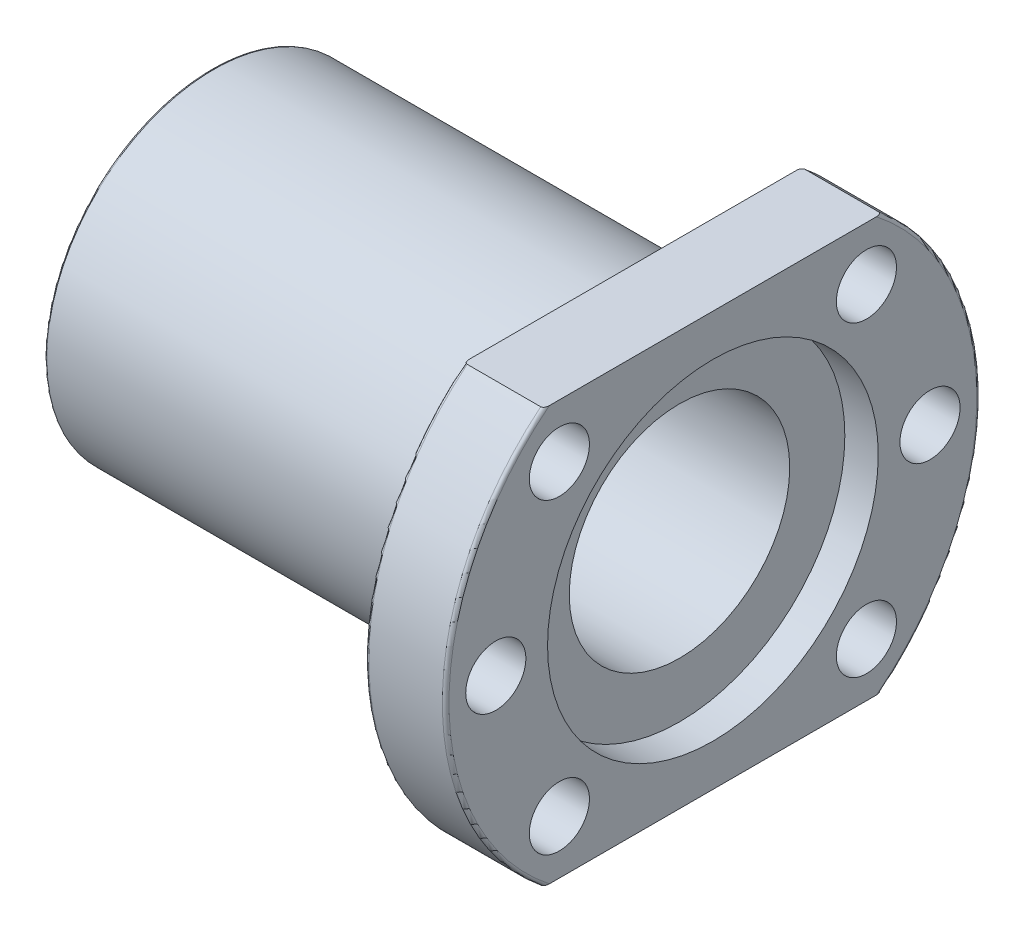
SolidWorks part; units mm, degrees
ref_plane "前视基准面" through (0, 0, 0) normal (0, 0, 1) x (1, 0, 0)
ref_plane "上视基准面" through (0, 0, 0) normal (0, 1, 0) x (1, 0, 0)
ref_plane "右视基准面" through (0, 0, 0) normal (1, 0, 0) x (0, 0, -1)
ref_plane "基准面4" through (-19.893, 0, 0) normal (1, 0, 0) x (0, 0, -1)
sketch "草图1" plane through (-19.893, 0, 0) normal (1, 0, 0) x (0, 0, -1)
  line L0 (25.2784, 31) -> (-25.2784, 31)
  line L1 (-25.2784, -31) -> (25.2784, -31)
  arc A0 (-25.2784, 31) -> (-25.2784, -31) centre (0, 0) ccw
  arc A1 (25.2784, -31) -> (25.2784, 31) centre (0, 0) ccw
extrude "凸台-拉伸1" add sketch "草图1" against normal blind 12
sketch "草图2" plane through (0, 0, 0) normal (0, 0, 1) x (1, 0, 0)
  line L0 (-94.893, 25) -> (-94.893, 0)
  line L1 (-94.893, 0) -> (-31.893, 0)
  line L2 (-31.893, 0) -> (-31.893, 25)
  line L3 (-31.893, 25) -> (-94.893, 25)
  line L4 (-94.893, 0) -> (-31.893, 0) construction
revolve "旋转1" add sketch "草图2" angle 360 about L4
hole_wizard "Ø9.0 (9) 直径孔1" positions "草图4" profile "草图3" hole size "Ø9.0" standard "ANSI Metric"
sketch "草图4" plane through (-31.893, 0, 0) normal (-1, 0, 0) x (0, 0, 1)
  point P0 (22.981, 22.981)
  point P1 (22.981, -22.981)
  point P2 (-22.981, -22.981)
  point P3 (-22.981, 22.981)
  point P4 (32.5, 0)
  point P5 (-32.5, 0)
sketch "草图3" plane through (-31.893, 22.981, 22.981) normal (0, 1, 0) x (0, 0, 1)
  line L0 (0, 0) -> (0, 12)
  line L1 (0, 12) -> (4.5, 12)
  line L2 (4.5, 12) -> (4.5, 0)
  line L5 (4.5, 0) -> (0, 0)
  line L11 (0, -6.35) -> (0, 107.95) construction
  dimension "通孔孔直径" = 9
  dimension "通孔孔深度" = 12
hole_wizard "M30 六角头螺栓的柱形沉头孔1" positions "草图6" profile "草图5" counterbore size "M30" standard "ANSI Metric"
sketch "草图6" plane through (-19.893, 0, 0) normal (1, 0, 0) x (0, 0, -1)
  point P0 (0, 0)
sketch "草图5" plane through (-19.893, 0, 0) normal (0, 1, 0) x (0, 0, -1)
  line L0 (0, 0) -> (0, 75)
  line L1 (0, 75) -> (16.5, 75)
  line L3 (16.5, 75) -> (16.5, 5)
  line L4 (16.5, 5) -> (24.75, 5)
  line L5 (24.75, 5) -> (24.75, 0)
  line L7 (24.75, 0) -> (0, 0)
  line L11 (0, -6.35) -> (0, 107.95) construction
  dimension "通孔孔直径" = 33
  dimension "通孔孔深度" = 75
  dimension "柱形沉头孔直径" = 49.5
  dimension "柱形沉头孔深度" = 5
fillet "圆角1" radius 0.3 1 edges at (-94.893, 0, -25)
fillet "圆角2" radius 0.5 4 edges at (-31.893, 0, 40) (-19.893, 0, 40) (-19.893, 0, -40) (-31.893, 0, -40)
